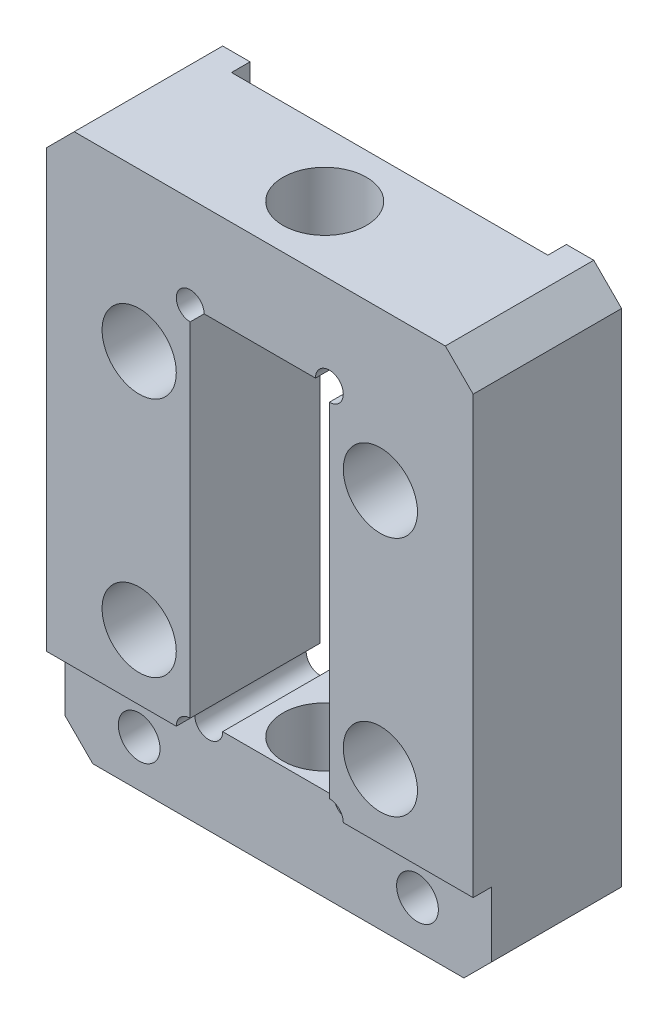
from build123d import *

# Parameters (mm, degrees)
SKETCH_1_W                  = 46
SKETCH_1_H                  = 60
EXTRUDE_1_DEPTH             = 8
SKETCH_19_W                 = 142.956519272
SKETCH_19_H                 = 61.410899124
CUT_EXTRUDE_7_DEPTH         = 2
SKETCH_21_W                 = 15
SKETCH_21_H                 = 40
CUT_EXTRUDE_9_DEPTH         = 42.048751504
HOLE_WIZARD_3_0_3_1_D       = 3
HOLE_WIZARD_9_0_9_1_D       = 9
SKETCH_26_W                 = 34.1
SKETCH_26_H                 = 84.411850982
CUT_EXTRUDE_10_DEPTH        = 2
HOLE_WIZARD_3_D             = 4.5
HOLE_WIZARD_3_CBORE_D       = 8
HOLE_WIZARD_3_CBORE_DEPTH   = 7
HOLE_WIZARD_3_2_D           = 4.2
HOLE_WIZARD_3_2_CBORE_D     = 8
HOLE_WIZARD_3_2_CBORE_DEPTH = 7
CHAMFER_2_SIZE              = 3
CHAMFER_1_SIZE              = 3


with BuildPart() as part:
    # 草图1 → 凸台-拉伸1 (new, symmetric)
    with BuildSketch(Plane.XY):
        Rectangle(SKETCH_1_W, SKETCH_1_H)
    extrude(amount=EXTRUDE_1_DEPTH, both=True)

    # 草图19 → 切除-拉伸7 (cut)
    with BuildSketch(Plane.XY.offset(8)):
        with Locations((33.235030531, -50.705449562)):
            Rectangle(SKETCH_19_W, SKETCH_19_H)
    extrude(amount=-CUT_EXTRUDE_7_DEPTH, mode=Mode.SUBTRACT)

    # 草图21 → 切除-拉伸9 (cut, through all)
    with BuildSketch(Plane.XY.offset(8)):
        Rectangle(SKETCH_21_W, SKETCH_21_H)
    extrude(amount=-CUT_EXTRUDE_9_DEPTH, mode=Mode.SUBTRACT)

    # Ø3.0 (3) 直径孔1 (through all)
    with Locations(Plane.XY.offset(8)):
        with Locations((-7.5, 20), (7.5, 20), (-7.5, -20), (7.5, -20)):
            Hole(HOLE_WIZARD_3_0_3_1_D / 2)

    # Ø9.0 (9) 直径孔1 (through all)
    with Locations(Plane(origin=(0, 30, 0), x_dir=(1, 0, 0), z_dir=(0, 1, 0))):
        with Locations((0, -1)):
            Hole(HOLE_WIZARD_9_0_9_1_D / 2)

    # 草图26 → 切除-拉伸10 (cut)
    with BuildSketch(Plane(origin=(0, 0, -8), x_dir=(-1, 0, 0), z_dir=(0, 0, -1))):
        Rectangle(SKETCH_26_W, SKETCH_26_H)
    extrude(amount=-CUT_EXTRUDE_10_DEPTH, mode=Mode.SUBTRACT)

    # Hole Wizard 3 (through all)
    with Locations(Plane(origin=(0, 0, -8), x_dir=(-1, 0, 0), z_dir=(0, 0, -1))):
        with Locations((-15, -25), (15, -25)):
            CounterBoreHole(HOLE_WIZARD_3_D / 2, HOLE_WIZARD_3_CBORE_D / 2, HOLE_WIZARD_3_CBORE_DEPTH)

    # Hole Wizard 3 2 (through all)
    with Locations(Plane.XY.offset(8)):
        with Locations((-13, 13), (13, 13), (-13, -13), (13, -13)):
            CounterBoreHole(HOLE_WIZARD_3_2_D / 2, HOLE_WIZARD_3_2_CBORE_D / 2, HOLE_WIZARD_3_2_CBORE_DEPTH)

    # 倒角2
    chamfer_2_edges = [part.edges().sort_by_distance(p)[0] for p in [
        (-23, 30, 0),
        (23, 30, 0),
    ]]
    chamfer(chamfer_2_edges, length=CHAMFER_2_SIZE)

    # 倒角1
    chamfer_1_edges = [part.edges().sort_by_distance(p)[0] for p in [
        (23, -30, -1),
        (-23, -30, -1),
    ]]
    chamfer(chamfer_1_edges, length=CHAMFER_1_SIZE)


solid = part.part
